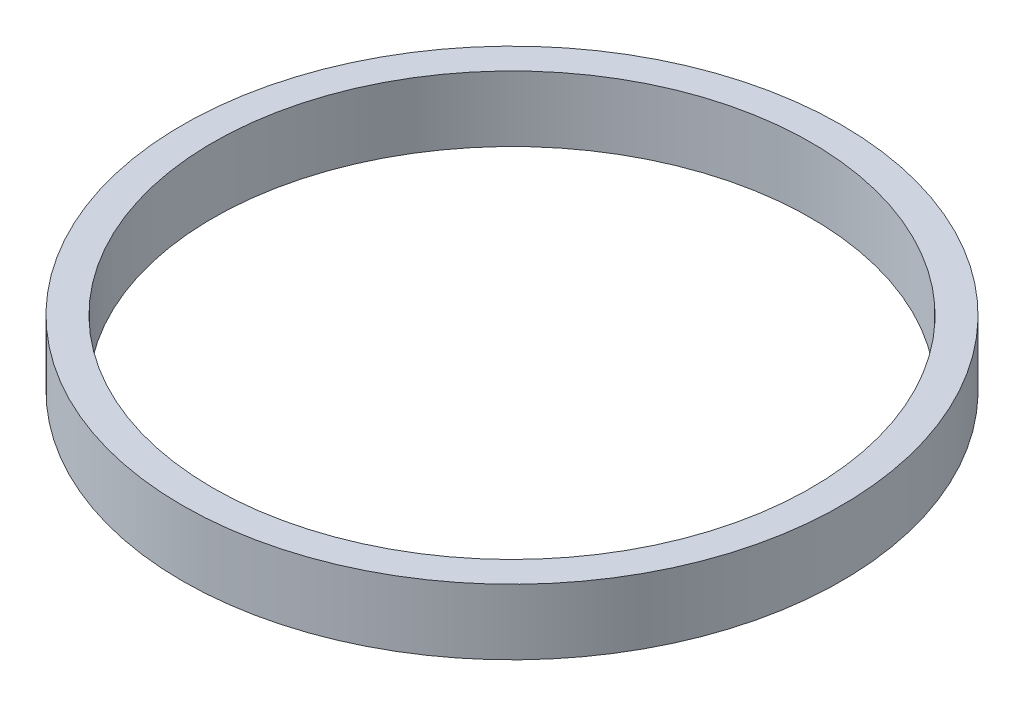
SolidWorks part; units mm, degrees
ref_plane "Front Plane" through (0, 0, 0) normal (0, 0, 1) x (1, 0, 0)
ref_plane "Top Plane" through (0, 0, 0) normal (0, 1, 0) x (1, 0, 0)
ref_plane "Right Plane" through (0, 0, 0) normal (1, 0, 0) x (0, 0, -1)
sketch "Sketch1" plane through (0, 0, 0) normal (0, 0, 1) x (1, 0, 0)
  line L0 (0, 0) -> (0, -35.6296) construction
  line L4 (70.4957, 151.5) -> (63.9957, 151.5)
  line L5 (70.4957, 151.5) -> (70.4957, 137.5)
  line L6 (70.4957, 137.5) -> (63.9957, 137.5)
  line L7 (63.9957, 151.5) -> (63.9957, 137.5)
  line L8 (-70.4957, 137.5) -> (70.4957, 137.5) construction
revolve "Revolve1" add sketch "Sketch1" angle 360 about L0
